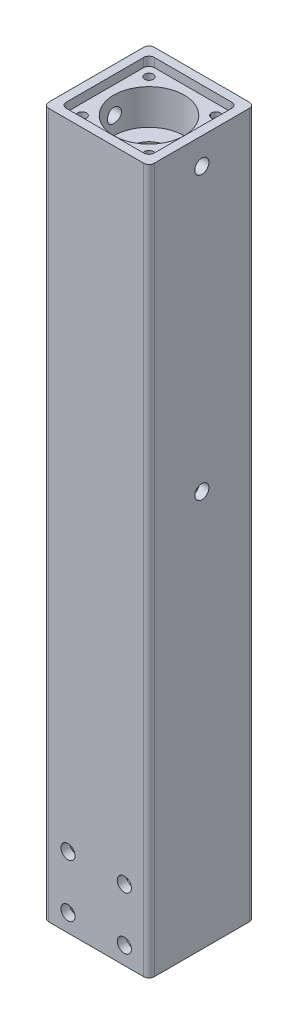
from build123d import *

# Parameters (mm, degrees)
SKETCH1_W               = 60
SKETCH1_H               = 60
BOSS_EXTRUDE1_DEPTH     = 400
SKETCH2_W               = 50
SKETCH2_H               = 50
CUT_EXTRUDE1_DEPTH      = 5
SKETCH3_R               = 20
CUT_EXTRUDE2_DEPTH      = 20
SKETCH4_R               = 10
CUT_EXTRUDE3_DEPTH      = 15
FILLET1_R               = 3
CUT_EXTRUDE4_DEPTH      = 30
CUT_EXTRUDE4_DEPTH_BACK = 30
SKETCH5_R               = 4
SKETCH6_W               = 50
SKETCH6_H               = 50
CUT_EXTRUDE5_DEPTH      = 60
SKETCH7_R               = 25
CUT_EXTRUDE6_DEPTH      = 300
CUT_EXTRUDE7_DEPTH      = 30
CUT_EXTRUDE7_DEPTH_BACK = 30
SKETCH8_R               = 4
CUT_EXTRUDE9_DEPTH      = 30
CUT_EXTRUDE9_DEPTH_BACK = 30
SKETCH10_R              = 4
FILLET2_R               = 3
SKETCH11_R              = 2.5
CUT_EXTRUDE11_DEPTH     = 20


with BuildPart() as part:
    # Sketch1 → Boss-Extrude1 (new body)
    with BuildSketch(Plane(origin=(0, 0, 0), x_dir=(1, 0, 0), z_dir=(0, 1, 0))):
        Rectangle(SKETCH1_W, SKETCH1_H)
    extrude(amount=BOSS_EXTRUDE1_DEPTH)

    # Sketch2 → Cut-Extrude1 (cut)
    with BuildSketch(Plane(origin=(0, 400, 0), x_dir=(1, 0, 0), z_dir=(0, 1, 0))):
        Rectangle(SKETCH2_W, SKETCH2_H)
    extrude(amount=-CUT_EXTRUDE1_DEPTH, mode=Mode.SUBTRACT)

    # Sketch3 → Cut-Extrude2 (cut)
    with BuildSketch(Plane(origin=(0, 395, 0), x_dir=(1, 0, 0), z_dir=(0, 1, 0))):
        with Locations(Location((0, 0, 0), (0, 0, 270))):
            Circle(SKETCH3_R)
    extrude(amount=-CUT_EXTRUDE2_DEPTH, mode=Mode.SUBTRACT)

    # Sketch4 → Cut-Extrude3 (cut)
    with BuildSketch(Plane(origin=(0, 375, 0), x_dir=(1, 0, 0), z_dir=(0, 1, 0))):
        with Locations(Location((0, 0, 0), (0, 0, 270))):
            Circle(SKETCH4_R)
    extrude(amount=-CUT_EXTRUDE3_DEPTH, mode=Mode.SUBTRACT)

    # Fillet1
    fillet1_edges = [part.edges().sort_by_distance(p)[0] for p in [
        (-30, 200, -30),
        (-30, 200, 30),
        (30, 200, 30),
        (30, 200, -30),
    ]]
    fillet(fillet1_edges, radius=FILLET1_R)

    # Sketch5 → Cut-Extrude4 (cut, two sides: drawn at the far end of the back side and taken through both)
    with BuildSketch(Plane(origin=(0, 0, 0), x_dir=(0, 0, -1), z_dir=(1, 0, 0)).offset(-CUT_EXTRUDE4_DEPTH_BACK)):
        with Locations(Location((0, 385, 0), (0, 0, 180))):
            Circle(SKETCH5_R)
    extrude(amount=CUT_EXTRUDE4_DEPTH + CUT_EXTRUDE4_DEPTH_BACK, mode=Mode.SUBTRACT)

    # Sketch6 → Cut-Extrude5 (cut)
    with BuildSketch(Plane.XZ):
        Rectangle(SKETCH6_W, SKETCH6_H)
    extrude(amount=-CUT_EXTRUDE5_DEPTH, mode=Mode.SUBTRACT)

    # Sketch7 → Cut-Extrude6 (cut)
    with BuildSketch(Plane.XZ.offset(-60)):
        with Locations(Location((0, 0, 0), (0, 0, 270))):
            Circle(SKETCH7_R)
    extrude(amount=-CUT_EXTRUDE6_DEPTH, mode=Mode.SUBTRACT)

    # Sketch8 → Cut-Extrude7 (cut, two sides: drawn at the far end of the back side and taken through both)
    with BuildSketch(Plane(origin=(0, 0, 0), x_dir=(0, 0, -1), z_dir=(1, 0, 0)).offset(-CUT_EXTRUDE7_DEPTH_BACK)):
        with Locations(Location((0, 225, 0), (0, 0, 180))):
            Circle(SKETCH8_R)
    extrude(amount=CUT_EXTRUDE7_DEPTH + CUT_EXTRUDE7_DEPTH_BACK, mode=Mode.SUBTRACT)

    # Sketch10 → Cut-Extrude9 (cut, two sides: drawn at the far end of the back side and taken through both)
    with BuildSketch(Plane.XY.offset(-CUT_EXTRUDE9_DEPTH_BACK)):
        with Locations((-16, 40)):
            Circle(SKETCH10_R)
        with Locations((-16, 10)):
            Circle(SKETCH10_R)
        with Locations(Location((16, 10, 0), (0, 0, 180))):
            Circle(SKETCH10_R)
        with Locations(Location((16, 40, 0), (0, 0, 180))):
            Circle(SKETCH10_R)
    extrude(amount=CUT_EXTRUDE9_DEPTH + CUT_EXTRUDE9_DEPTH_BACK, mode=Mode.SUBTRACT)

    # Fillet2
    fillet2_edges = [part.edges().sort_by_distance(p)[0] for p in [
        (25, 397.5, -25),
        (25, 397.5, 25),
        (-25, 397.5, 25),
        (-25, 397.5, -25),
    ]]
    fillet(fillet2_edges, radius=FILLET2_R)

    # Sketch11 → Cut-Extrude11 (cut)
    with BuildSketch(Plane(origin=(0, 395, 0), x_dir=(1, 0, 0), z_dir=(0, 1, 0))):
        with Locations(Location((-19, 19, 0), (0, 0, 270))):
            Circle(SKETCH11_R)
        with Locations(Location((19, 19, 0), (0, 0, 270))):
            Circle(SKETCH11_R)
        with Locations(Location((-19, -19, 0), (0, 0, 270))):
            Circle(SKETCH11_R)
        with Locations(Location((19, -19, 0), (0, 0, 270))):
            Circle(SKETCH11_R)
    extrude(amount=-CUT_EXTRUDE11_DEPTH, mode=Mode.SUBTRACT)


solid = part.part
